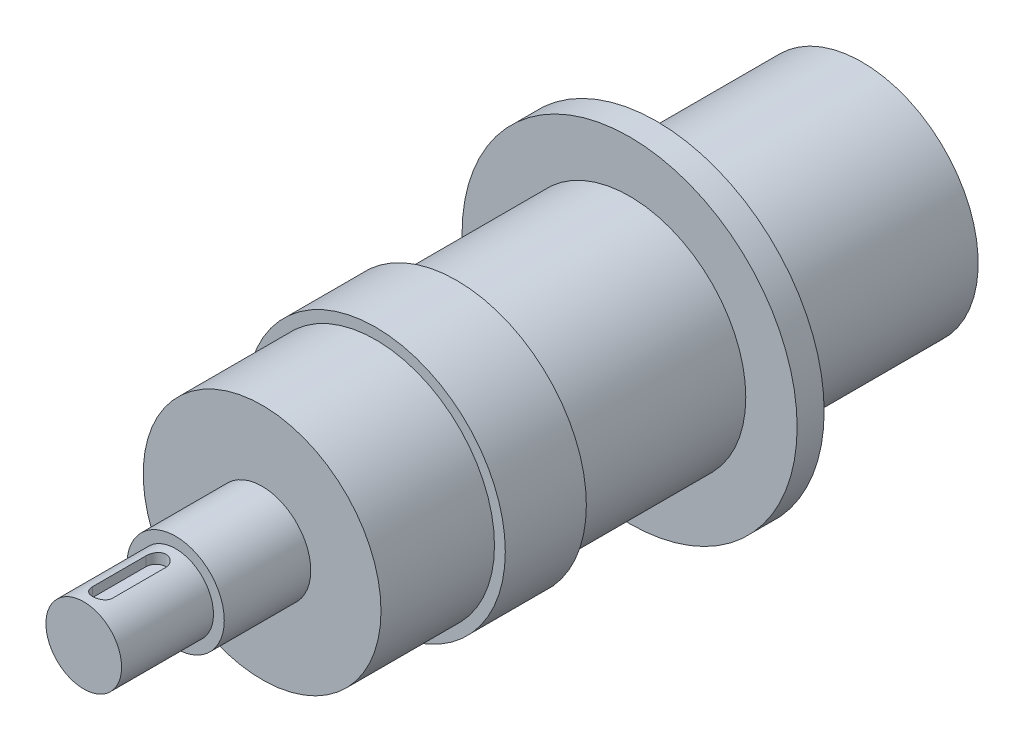
from build123d import *

# Parameters (mm, degrees)
SKETCH1_R             = 21.5
BOSS_EXTRUDE1_DEPTH   = 37
SKETCH2_R             = 24
BOSS_EXTRUDE2_DEPTH   = 15
SKETCH3_R             = 22
BOSS_EXTRUDE3_DEPTH   = 21
SKETCH4_R             = 9
BOSS_EXTRUDE4_DEPTH   = 16
SKETCH5_R             = 7
BOSS_EXTRUDE5_DEPTH   = 17
CUT_EXTRUDE1_START    = 30
CUT_EXTRUDE1_DEPTH    = 25
BOSS_EXTRUDE6_START   = 38
SKETCH7_R             = 21.5
BOSS_EXTRUDE6_DEPTH   = 38
SKETCH9_R             = 31
BOSS_EXTRUDE7_DEPTH   = 5
M8_TAPPED_HOLE1_D     = 6.8
M8_TAPPED_HOLE1_DEPTH = 35
M8_TAPPED_HOLE1_TIP   = 2.042926105


with BuildPart() as part:
    # Sketch1 → Boss-Extrude1 (new body)
    with BuildSketch(Plane.XY.offset(38)):
        Circle(SKETCH1_R)
    extrude(amount=BOSS_EXTRUDE1_DEPTH)

    # Sketch2 → Boss-Extrude2 (add)
    with BuildSketch(Plane.XY.offset(75)):
        Circle(SKETCH2_R)
    extrude(amount=BOSS_EXTRUDE2_DEPTH)

    # Sketch3 → Boss-Extrude3 (add)
    with BuildSketch(Plane.XY.offset(90)):
        Circle(SKETCH3_R)
    extrude(amount=BOSS_EXTRUDE3_DEPTH)

    # Sketch4 → Boss-Extrude4 (add)
    with BuildSketch(Plane.XY.offset(111)):
        Circle(SKETCH4_R)
    extrude(amount=BOSS_EXTRUDE4_DEPTH)

    # Sketch5 → Boss-Extrude5 (add)
    with BuildSketch(Plane.XY.offset(127)):
        Circle(SKETCH5_R)
    extrude(amount=BOSS_EXTRUDE5_DEPTH)

    # Sketch6 → Cut-Extrude1 (cut)
    with BuildSketch(Plane(origin=(0, 0, 0), x_dir=(1, 0, 0), z_dir=(0, 1, 0)).offset(CUT_EXTRUDE1_START)):
        with BuildLine():
            Line((1.85, -130.63993085), (1.85, -140.5))
            ThreePointArc((1.85, -140.5), (0, -142.35), (-1.85, -140.5))
            Line((-1.85, -140.5), (-1.85, -130.63993085))
            ThreePointArc((-1.85, -130.63993085), (0, -128.78993085), (1.85, -130.63993085))
        make_face()
    extrude(amount=-CUT_EXTRUDE1_DEPTH, mode=Mode.SUBTRACT)

    # Sketch7 → Boss-Extrude6 (add)
    with BuildSketch(Plane(origin=(0, 0, 38), x_dir=(-1, 0, 0), z_dir=(0, 0, -1)).offset(BOSS_EXTRUDE6_START)):
        Circle(SKETCH7_R)
    extrude(amount=-BOSS_EXTRUDE6_DEPTH)

    # Sketch9 → Boss-Extrude7 (add)
    with BuildSketch(Plane.XY.offset(38)):
        Circle(SKETCH9_R)
    extrude(amount=BOSS_EXTRUDE7_DEPTH)

    # M8 Tapped Hole1
    with Locations(Plane(origin=(0, 0, 0), x_dir=(-1, 0, 0), z_dir=(0, 0, -1))):
        with Locations((0, 0)):
            Hole(M8_TAPPED_HOLE1_D / 2, depth=M8_TAPPED_HOLE1_DEPTH)
            with Locations((0, 0, -(M8_TAPPED_HOLE1_DEPTH + M8_TAPPED_HOLE1_TIP / 2))):  # 118° drill point
                Cone(0, M8_TAPPED_HOLE1_D / 2, M8_TAPPED_HOLE1_TIP, mode=Mode.SUBTRACT)


solid = part.part
